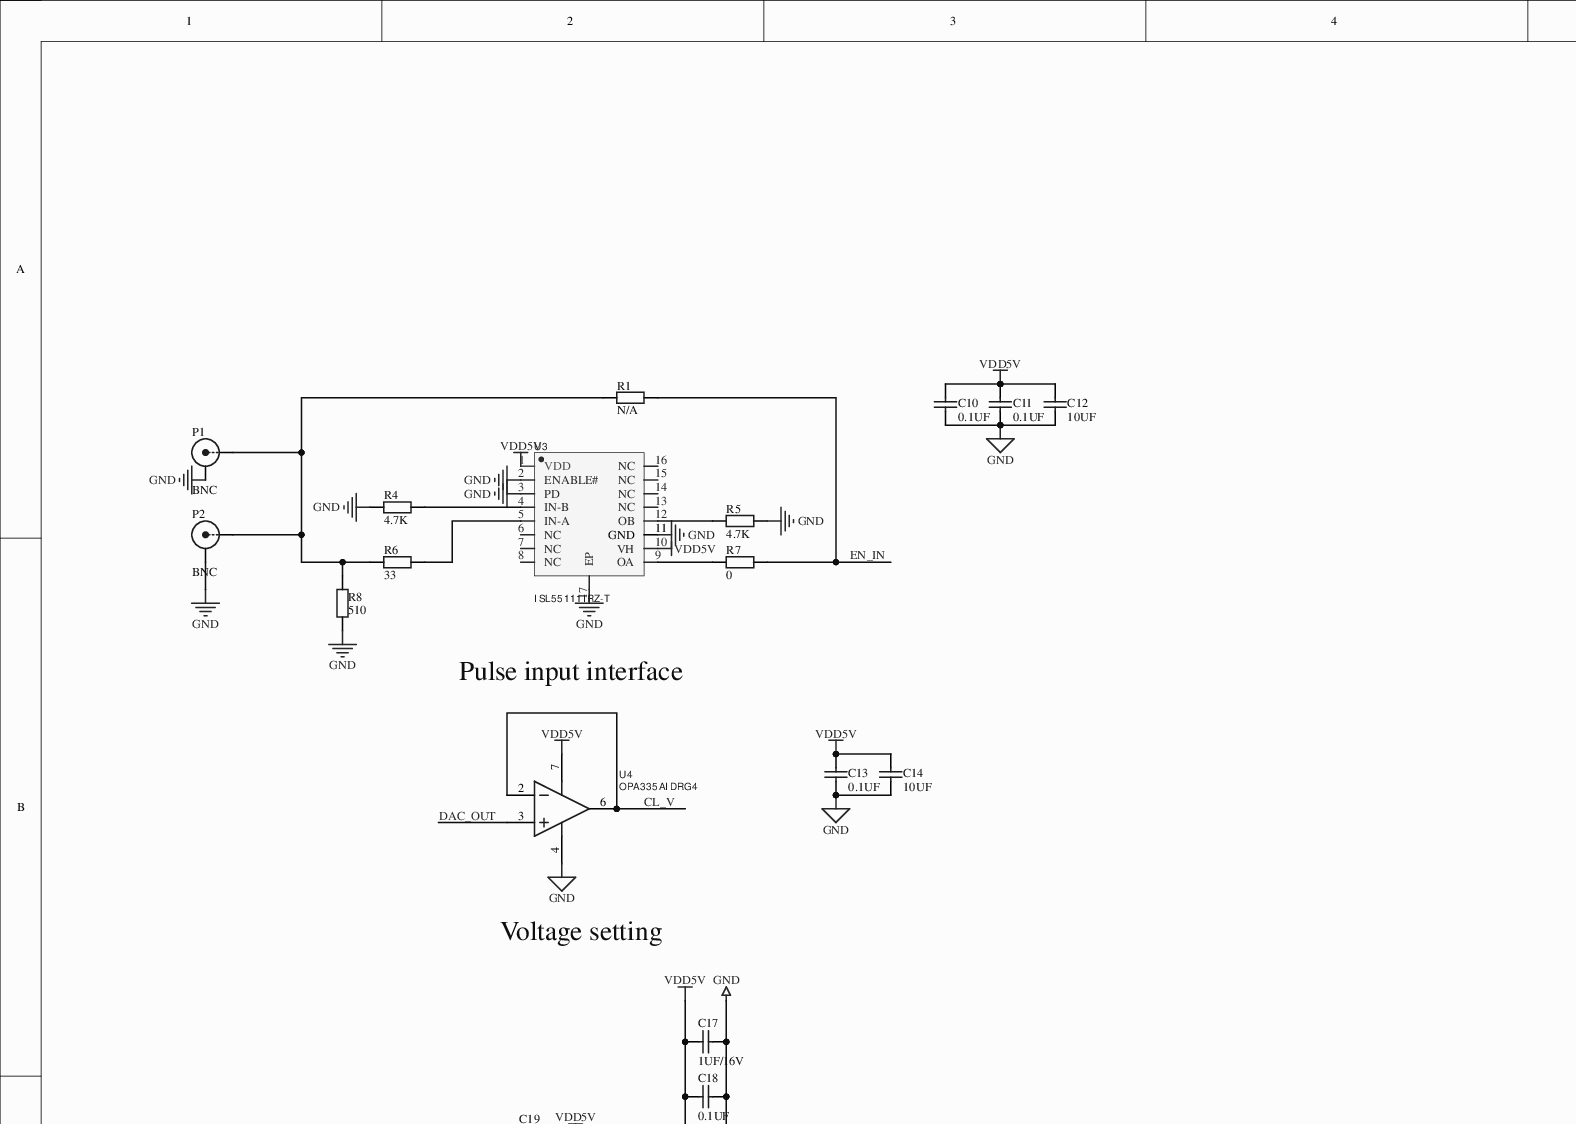
[diagram p0: MISC80814-4.SchDoc, top left]
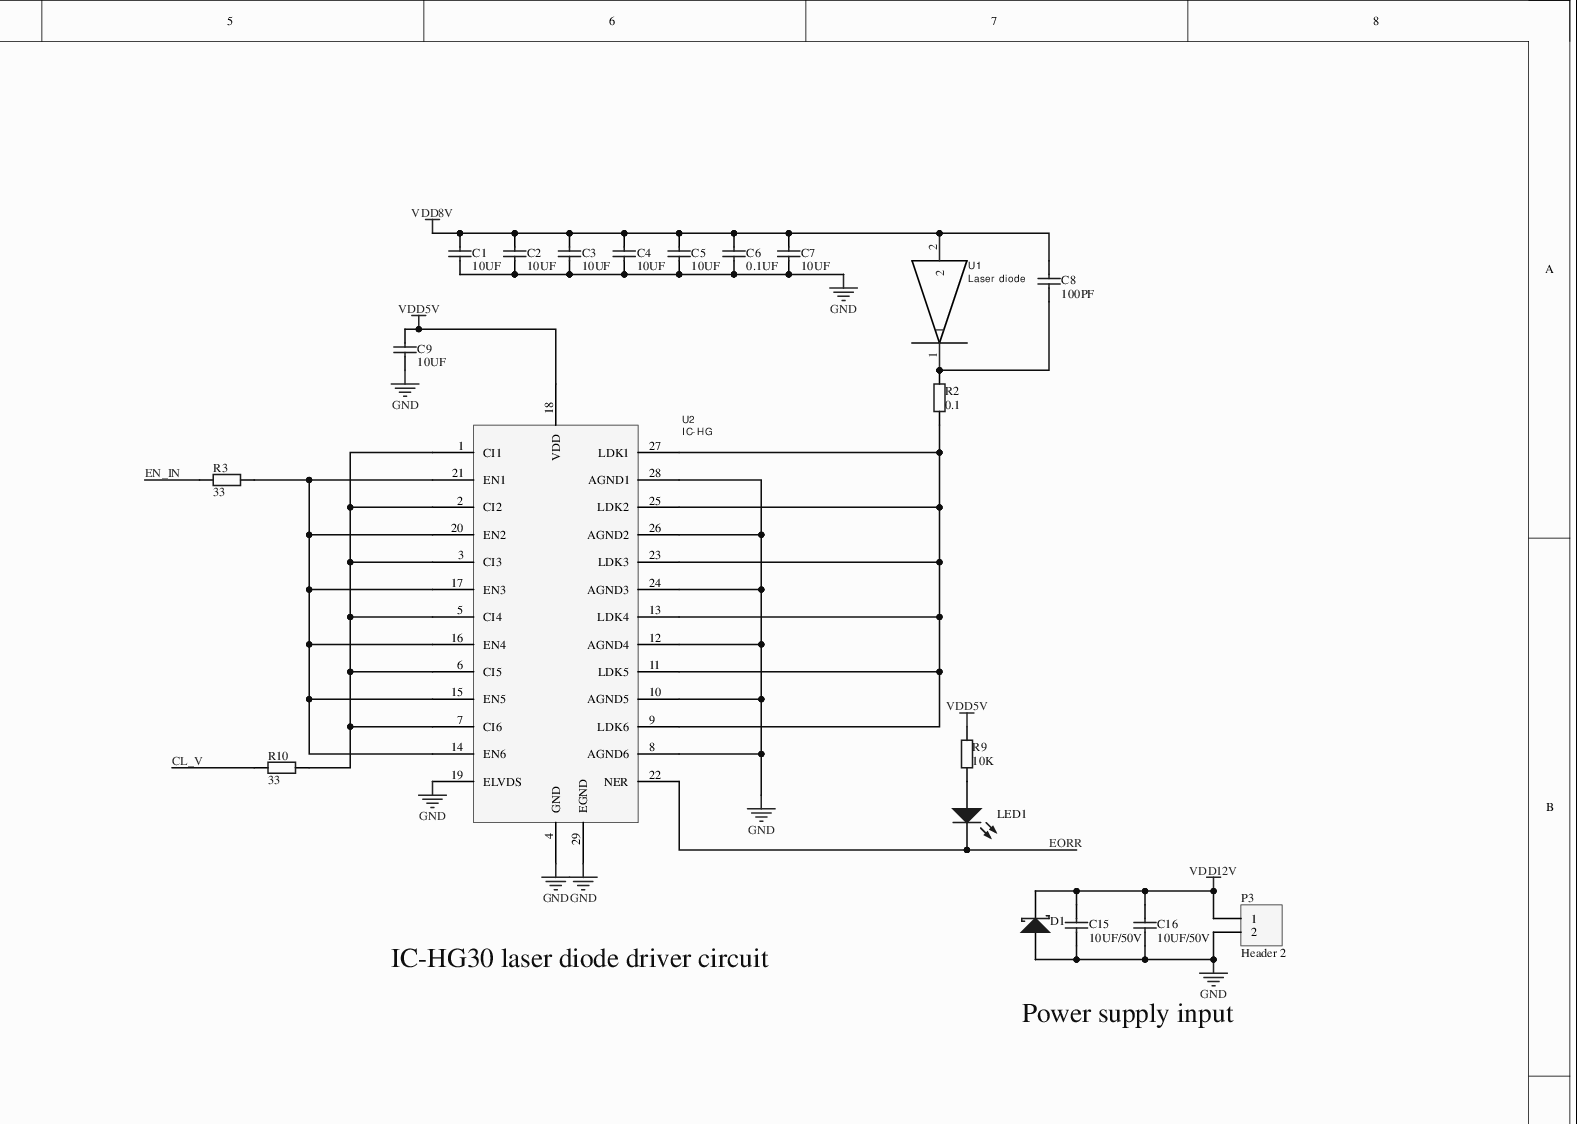
[diagram p1: MISC80814-4.SchDoc, top right]
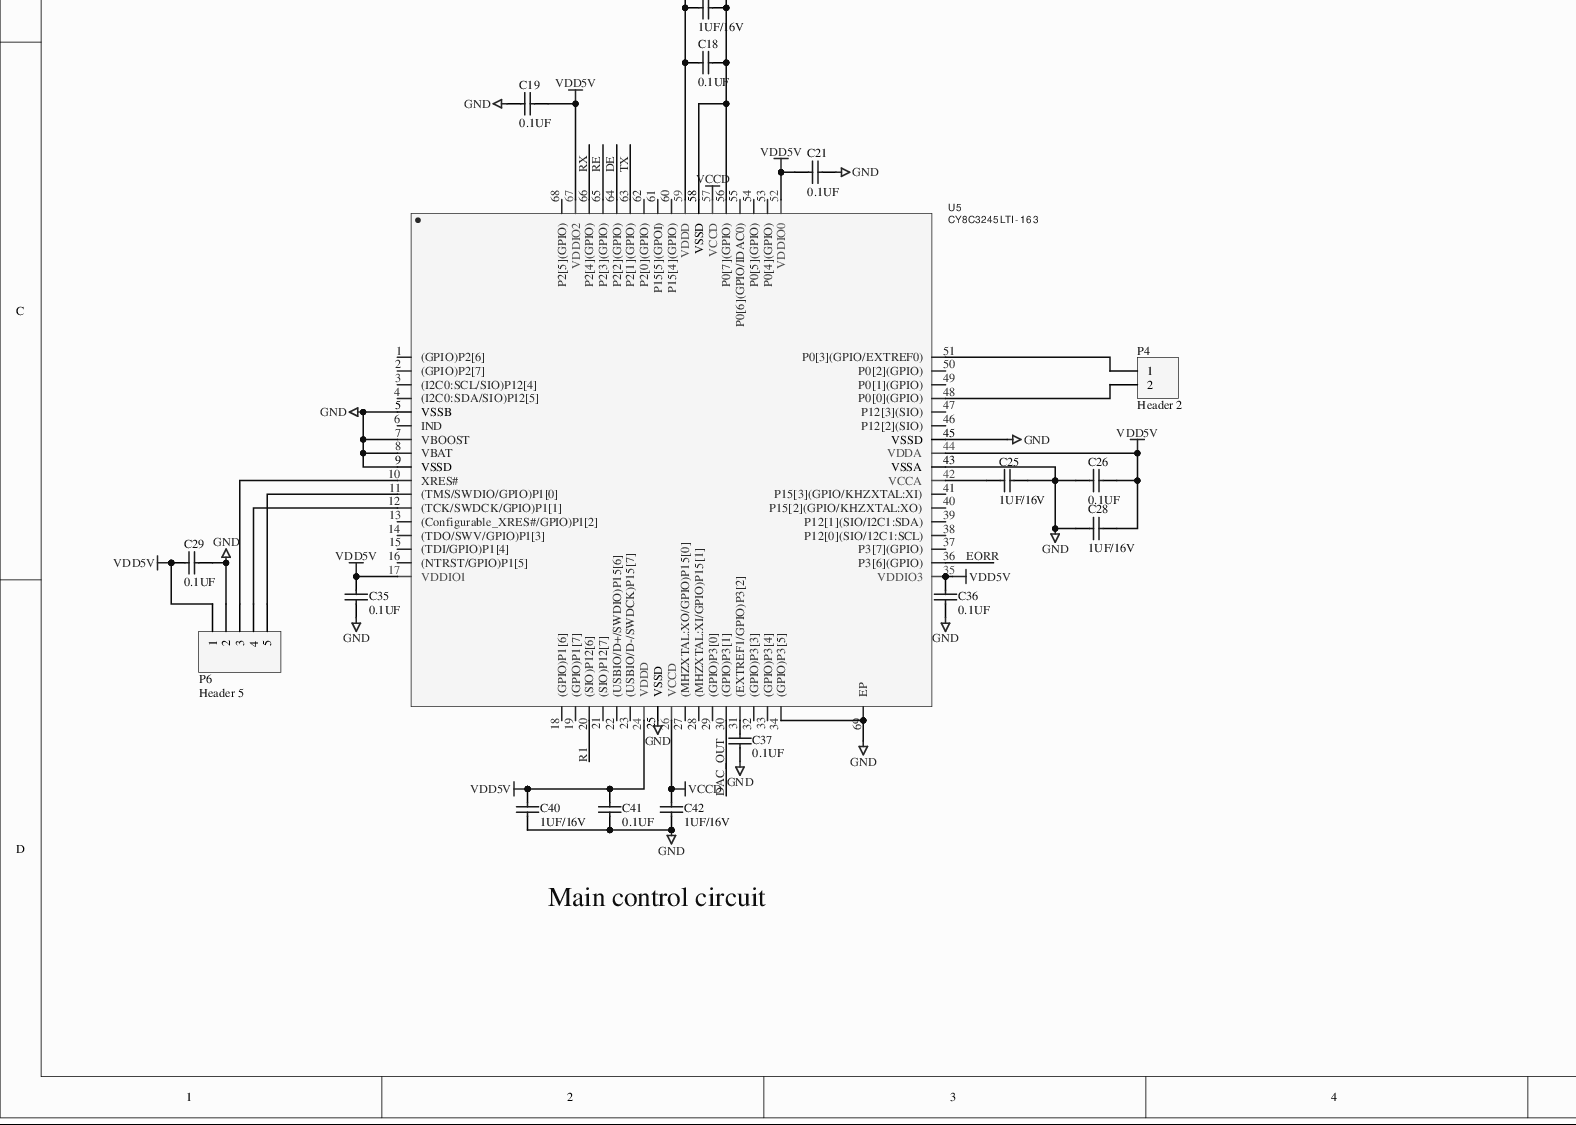
[diagram p2: MISC80814-4.SchDoc, bottom left]
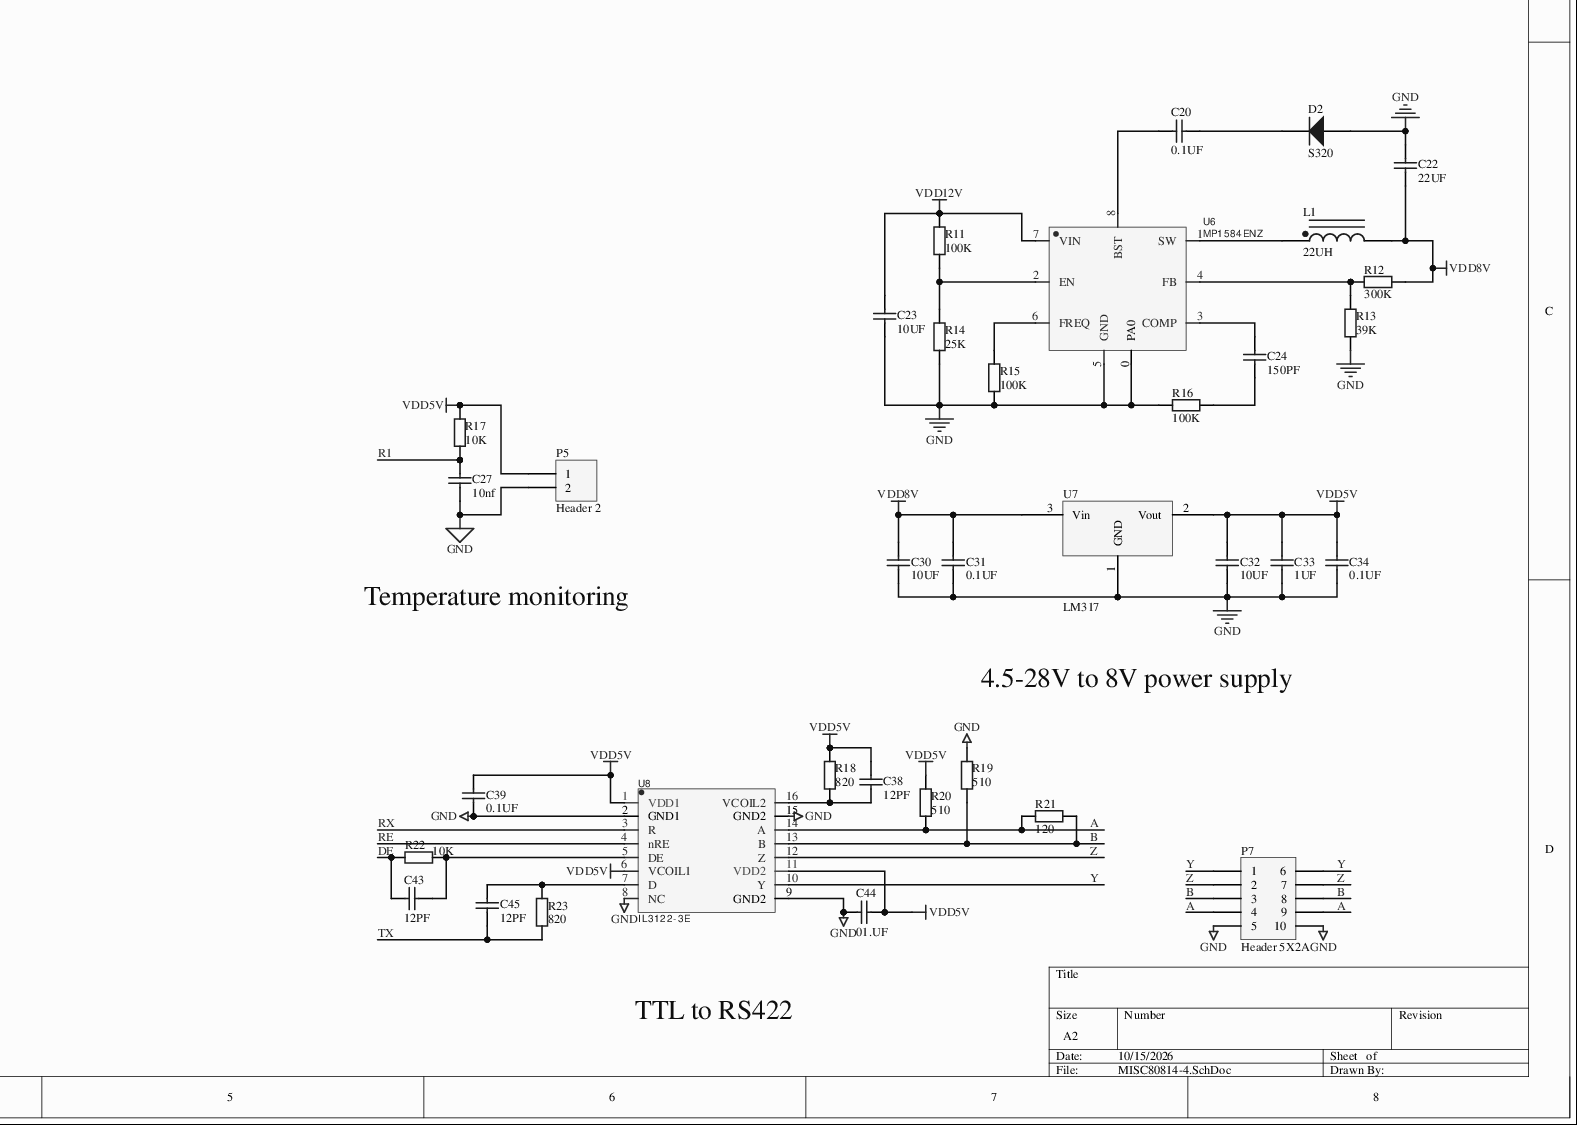
[diagram p3: MISC80814-4.SchDoc, bottom right]
# Altium project MISC80814-7.PrjPcb
1 sheet, 87 parts. Net scope: global (net labels, ports and power ports of the same name join across sheets).
Board file: MISC80814.PcbDoc

## Sheet MISC80814-4.SchDoc
size A2

### Parts
C1  10UF  [C0603]
C2  10UF  [C0603]
C3  10UF  [C0603]
C4  10UF  [C0603]
C5  10UF  [C0603]
C6  0.1UF  [C0603]
C7  10UF  [C0603]
C8  100PF  [C0603]
C9  10UF  [C0603]
C10  0.1UF  [C0603]
C11  0.1UF  [C0603]
C12  10UF  [C0603]
C13  0.1UF  [C0603]
C14  10UF  [C0603]
C15  10UF/50V  [C1206]
C16  10UF/50V  [C1206]
C17  1UF/16V  [C1206]
C18  0.1UF  [C0603]
C19  0.1UF  [C0603]
C20  0.1UF  [C0603]
C21  0.1UF  [C0603]
C22  22UF  [C0603]
C23  10UF  [C0603]
C24  150PF  [C0603]
C25  1UF/16V  [C1206]
C26  0.1UF  [C0603]
C27  10nf  [C0603]
C28  1UF/16V  [C1206]
C29  0.1UF  [C0603]
C30  10UF  [C0603]
C31  0.1UF  [C0603]
C32  10UF  [C0603]
C33  1UF  [C0603]
C34  0.1UF  [C0603]
C35  0.1UF  [C0603]
C36  0.1UF  [C0603]
C37  0.1UF  [C0603]
C38  12PF  [C0603]
C39  0.1UF  [C0603]
C40  1UF/16V  [C1206]
C41  0.1UF  [C0603]
C42  1UF/16V  [C1206]
C43  12PF  [C0603]
C44  01.UF  [C0603]
C45  12PF  [C0603]
D1  D Schottky  [SMB]  (value not drawn)
D2  S320  [SMC]
L1  22UH  [DIODE_SMC]
LED1  LED2  [3.2X1.6X1.1]  (value not drawn)
P1  BNC  [BNC_RA CON]
P2  BNC  [BNC_RA CON]
P3  Header 2  [HDR1X2]
P4  Header 2  [HDR1X2]
P5  Header 2  [HDR1X2]
P6  Header 5  [HDR1X5]
P7  Header 5X2A  [HDR2X5_CEN]
R1  N/A  [J1-0603]
R2  0.1  [J1-0603]
R3  33  [J1-0603]
R4  4.7K  [J1-0603]
R5  4.7K  [J1-0603]
R6  33  [J1-0603]
R7  0  [J1-0603]
R8  510  [J1-0603]
R9  10K  [J1-0603]
R10  33  [J1-0603]
R11  100K  [J1-0603]
R12  300K  [J1-0603]
R13  39K  [J1-0603]
R14  25K  [J1-0603]
R15  100K  [J1-0603]
R16  100K  [J1-0603]
R17  10K  [J1-0603]
R18  820  [J1-0603]
R19  510  [J1-0603]
R20  510  [J1-0603]
R21  120  [J1-0603]
R22  10K  [J1-0603]
R23  820  [J1-0603]
U1  Laser diode  [激光二极管]
U2  IC-HG  [QFN28-5X5]
U3  ISL55111IRZ-T  [QFN-16_L4.0-W4.0-P0.65-BL-EP2.6]
U4  OPA335AIDRG4  [SOP8]
U5  CY8C3245LTI-163  [QFN-68_L8.0-W8.0-P0.40-TL-EP5.7]
U6  MP1584ENZ  [MP1548EN]
U7  LM317  [TO220A]
U8  IL3122-3E  [SOIC-16_L9.9-W3.9-P1.27-LS6.0-BL]

### Nets
GND: C1.1 C2.1 C3.1 C4.1 C5.1 C6.1 C7.1 C9.1 C10.1 C11.1 C12.1 C13.1 C14.1 C15.1 C16.1 C17.1 C18.1 C19.2 C21.1 C22.1 C23.2 C25.1 C26.2 C27.2 C28.2 C29.2 C30.2 C31.2 C32.2 C33.2 C34.2 C35.1 C36.2 C37.2 C39.2 C40.2 C41.2 C42.2 C44.2 D1.1(A) D2.1(A) P1.2(Y) P2.2(Y) P3.2 P5.2 P6.2 P7.5 P7.10 R4.2 R5.1 R8.2 R13.2 R14.1 R15.1 R16.1 R19.1 U2.4(GND) U2.8(AGND6) U2.10(AGND5) U2.12(AGND4) U2.19(ELVDS) U2.24(AGND3) U2.26(AGND2) U2.28(AGND1) U2.29(EGND) U3.2(ENABLE#) U3.3(PD) U3.11(GND) U3.17(EP) U4.4(V-) U5.5(VSSB) U5.7(VBOOST) U5.8(VBAT) U5.9(VSSD) U5.25(VSSD) U5.34((GPIO)P3[5]) U5.43(VSSA) U5.45(VSSD) U5.56(P0[7](GPIO)) U5.58(VSSD) U5.69(EP) U6.0(PA0) U6.5(GND) U7.1(GND) U8.2(GND1) U8.8(NC) U8.9(GND2) U8.15(GND2)
VCCD: C42.1 U5.26(VCCD) U5.57(VCCD)
VDD5V: C9.2 C10.2 C11.2 C12.2 C13.2 C14.2 C17.2 C18.2 C19.1 C21.2 C26.1 C28.1 C29.1 C32.1 C33.1 C34.1 C35.2 C36.1 C38.2 C39.1 C40.1 C41.1 C44.1 P5.1 P6.1 R9.2 R17.2 R18.1 R20.1 U2.18(VDD) U3.1(VDD) U3.10(VH) U4.7(V+) U5.17(VDDIO1) U5.24(VDDD) U5.35(VDDIO3) U5.44(VDDA) U5.52(VDDIO0) U5.59(VDDD) U5.67(VDDIO2) U7.2(Vout) U8.1(VDD1) U8.6(VCOIL1) U8.11(VDD2)
VDD8V: C1.2 C2.2 C3.2 C4.2 C5.2 C6.2 C7.2 C8.2 C22.2 C30.1 C31.1 L1.2 R12.1 U1.2 U7.3(Vin)
VDD12V: C15.2 C16.2 C23.1 D1.2(K) P3.1 R11.2 U6.7(VIN)
A: P7.4 P7.9 R20.2 R21.1 U8.14(A)
B: P7.3 P7.8 R19.2 R21.2 U8.13(B)
CL_V: R10.2 U4.2(IN-) U4.6(OUT)
DAC_OUT: U4.3(IN+) U5.30((GPIO)P3[1])
DE: C43.1 R22.2 U5.64(P2[2](GPIO))
EN_IN: R1.1 R3.2 R7.1
EORR: LED1.2(K) U2.22(NER) U5.36(P3[6](GPIO))
R1: C27.1 R17.1 U5.20((SIO)P12[6])
RE: U5.65(P2[3](GPIO)) U8.4(nRE)
RX: U5.66(P2[4](GPIO)) U8.3(R)
TX: C45.1 R23.1 U5.63(P2[1](GPIO))
Y: P7.1 P7.6 U8.10(Y)
Z: P7.2 P7.7 U8.12(Z)
NetC8_1: C8.1 R2.2 U1.1
NetC20_1: C20.1 D2.2(K)
NetC20_2: C20.2 U6.8(BST)
NetC24_1: C24.1 U6.3(COMP)
NetC24_2: C24.2 R16.2
NetC25_2: C25.2 U5.42(VCCA)
NetC37_1: C37.1 U5.31((EXTREF1/GPIO)P3[2])
NetC38_1: C38.1 R18.2 U8.16(VCOIL2)
NetC43_2: C43.2 R22.1 U8.5(DE)
NetC45_2: C45.2 R23.2 U8.7(D)
NetL1_1: L1.1 U6.1(SW)
NetLED1_1: LED1.1(A) R9.1
NetP1_1: P1.1(X) P2.1(X) R1.2 R6.2 R8.1
NetP4_1: P4.1 U5.51(P0[3](GPIO/EXTREF0))
NetP4_2: P4.2 U5.48(P0[0](GPIO))
NetP6_3: P6.3 U5.10(XRES#)
NetP6_4: P6.4 U5.12((TCK/SWDCK/GPIO)P1[1])
NetP6_5: P6.5 U5.11((TMS/SWDIO/GPIO)P1[0])
NetR2_1: R2.1 U2.9(LDK6) U2.11(LDK5) U2.13(LDK4) U2.23(LDK3) U2.25(LDK2) U2.27(LDK1)
NetR3_1: R3.1 U2.14(EN6) U2.15(EN5) U2.16(EN4) U2.17(EN3) U2.20(EN2) U2.21(EN1)
NetR4_1: R4.1 U3.4(IN-B)
NetR5_2: R5.2 U3.12(OB)
NetR6_1: R6.1 U3.5(IN-A)
NetR7_2: R7.2 U3.9(OA)
NetR10_1: R10.1 U2.1(CI1) U2.2(CI2) U2.3(CI3) U2.5(CI4) U2.6(CI5) U2.7(CI6)
NetR11_1: R11.1 R14.2 U6.2(EN)
NetR12_2: R12.2 R13.1 U6.4(FB)
NetR15_2: R15.2 U6.6(FREQ)

Not connected (* = marked no-connect by the designer): U3 6(NC) 7(NC) 8(NC) 13(NC) 14(NC) 15(NC) 16(NC); U5 1((GPIO)P2[6]) 2((GPIO)P2[7]) 3((I2C0:SCL/SIO)P12[4]) 4((I2C0:SDA/SIO)P12[5]) 6(IND) 13((Configurable_XRES#/GPIO)P1[2]) 14((TDO/SWV/GPIO)P1[3]) 15((TDI/GPIO)P1[4]) 16((NTRST/GPIO)P1[5]) 18((GPIO)P1[6]) 19((GPIO)P1[7]) 21((SIO)P12[7]) 22((USBIO/D+/SWDIO)P15[6]) 23((USBIO/D-/SWDCK)P15[7]) 27((MHZXTAL:XO/GPIO)P15[0]) 28((MHZXTAL:XI/GPIO)P15[1]) 29((GPIO)P3[0]) 32((GPIO)P3[3]) 33((GPIO)P3[4]) 37(P3[7](GPIO)) 38(P12[0](SIO/12C1:SCL)) 39(P12[1](SIO/I2C1:SDA)) 40(P15[2](GPIO/KHZXTAL:XO)) 41(P15[3](GPIO/KHZXTAL:XI)) 46(P12[2](SIO)) 47(P12[3](SIO)) 49(P0[1](GPIO)) 50(P0[2](GPIO)) 53(P0[4](GPIO)) 54(P0[5](GPIO)) 55(P0[6](GPIO/IDAC0)) 60(P15[4](GPIO)) 61(P15[5](GPOI)) 62(P2[0](GPIO)) 68(P2[5](GPIO))

### Notes on the sheet
- Pulse input interface
- Voltage setting
- IC-HG30 laser diode driver circuit
- Power supply input
- Temperature monitoring
- 4.5-28V to 8V power supply
- Main control circuit
- TTL to RS422

### Library data of the parts
C1-C7 C9-C14 C18-C24 C26 C27 C29-C39 C41 C43-C45 = Cap Semi: Capacitor (Semiconductor SIM Model); Value: 100pF; Published: 8-Jun-2000; LatestRevisionDate: 29-May-2009; LatestRevisionNote: IPC-7351 Footprint Added.; PackageReference: C1206; PackageDescription: Chip Capacitor; Publisher: Altium Limited
C8 C15-C17 C25 C28 C40 C42 = Cap Semi: Capacitor (Semiconductor SIM Model); Published: 8-Jun-2000; LatestRevisionDate: 29-May-2009; LatestRevisionNote: IPC-7351 Footprint Added.; PackageReference: C1206; PackageDescription: Chip Capacitor; Publisher: Altium Limited
  C8: Value: 100pF
D1 = D Schottky: Schottky Diode; Published: 8-Jun-2000; LatestRevisionDate: 17-Jul-2002; LatestRevisionNote: Re-released for DXP Platform.; PackageReference: SMB; PackageDescription: DO-214-AA/SMB; 2 C-Bend Leads; Body 5.3 x 3.6 mm, inc. leads (LxW); Code_JEDEC: DO-214-AA; Publisher: Altium Limited
D2 = Diode: Default Diode; Published: 8-Jun-2000; LatestRevisionDate: 17-Jul-2002; LatestRevisionNote: Re-released for DXP Platform.; PackageVersion: Sep-1996; PackageReference: SMC; PackageDescription: DO-214-AB/SMC; 2 C-Bend Leads; Body 7.9 x 5.9 mm, inc. leads (LxW); Code_JEDEC: DO-214-AB; Publisher: Altium Limited
L1 = Inductor Iron Dot: Magnetic-Core Inductor with Winding Polarity Marking; Value: 10mH; Published: 24-Mar-1999; LatestRevisionDate: 17-Jul-2002; LatestRevisionNote: Re-released for DXP Platform.; PackageReference: DIODE_SMC; PackageDescription: Diode; 2 Leads; Publisher: Altium Limited
LED1 = LED2: Typical RED, GREEN, YELLOW, AMBER GaAs LED; Published: 8-Jun-2000; LatestRevisionDate: 17-Jul-2002; LatestRevisionNote: Re-released for DXP Platform.; PackageVersion: Feb-2002; PackageReference: 3.2X1.6X1.1; PackageDescription: SM LED; 2 Flat Leads; Publisher: Altium Limited
P1 P2 = BNC: BNC Elbow Connector; LatestRevisionDate: 17-Jul-2002; LatestRevisionNote: Re-released for DXP Platform.; Publisher: Altium Limited
P3-P5 = Header 2: Header, 2-Pin; LatestRevisionDate: 17-Jul-2002; LatestRevisionNote: Re-released for DXP Platform.; Publisher: Altium Limited
P6 = Header 5: Header, 5-Pin; LatestRevisionDate: 17-Jul-2002; LatestRevisionNote: Re-released for DXP Platform.; Publisher: Altium Limited
P7 = Header 5X2A: Header, 5-Pin, Dual row; LatestRevisionDate: 17-Jul-2002; LatestRevisionNote: Re-released for DXP Platform.; Publisher: Altium Limited
R1-R23 = Res2: Resistor; Value: 1K; Published: 8-Jun-2000; LatestRevisionDate: 17-Jul-2002; LatestRevisionNote: Re-released for DXP Platform.; PackageReference: AXIAL-0.4; PackageDescription: Axial Device, Thru-Hole; 2 Leads; 0.4 in Pin Spacing; Publisher: Altium Limited
U1 = 激光二极管
U6 = MP1584ENZ_own
U7 = LM317: Adjustable linear regulator IC